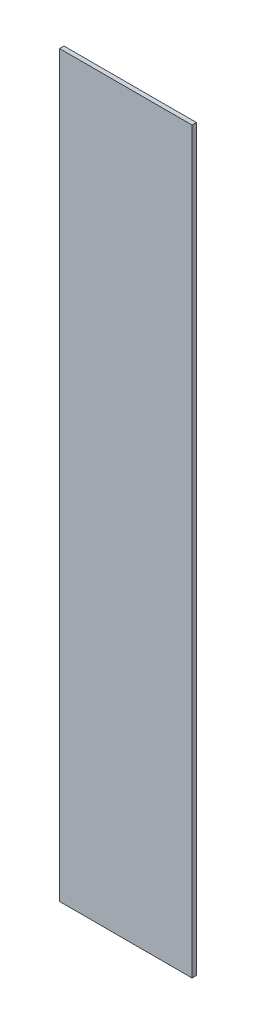
SolidWorks part; units mm, degrees
material "PMMA(有机玻璃)"
ref_plane "前视" through (0, 0, 0) normal (0, 0, 1) x (1, 0, 0)
ref_plane "上视" through (0, 0, 0) normal (0, 1, 0) x (1, 0, 0)
ref_plane "右视" through (0, 0, 0) normal (1, 0, 0) x (0, 0, -1)
sketch "草图1" plane through (0, 0, 0) normal (0, 0, 1) x (1, 0, 0)
  line L1 (-75.5, 421) -> (75.5, 421)
  line L2 (-75.5, 421) -> (-75.5, -421)
  line L3 (-75.5, -421) -> (75.5, -421)
  line L4 (75.5, 421) -> (75.5, -421)
  line L5 (-75.5, 421) -> (75.5, -421) construction
  line L6 (-75.5, -421) -> (75.5, 421) construction
  point P0 (0, 0)
  dimension "D1" = 842
  dimension "D2" = 151
extrude "凸台-拉伸1" add sketch "草图1" along normal blind 5
hole_wizard "M5 间隙孔1" positions "草图3" profile "草图2" hole size "M5" standard "GB"
sketch "草图3" plane through (0, 0, 5) normal (0, 0, 1) x (1, 0, 0)
  line L0 (-427.5, 273) -> (-427.5, -273) construction
  line L1 (-427.5, -273) -> (427.5, -273) construction
  line L2 (0, 273) -> (0, -273) construction
  line L3 (427.5, 273) -> (-427.5, 273) construction
  line L5 (-427.5, 0) -> (427.5, 0) construction
  line L6 (427.5, -273) -> (427.5, 273) construction
  point P0 (-375, -261)
  point P46 (415.5, 250)
  point P48 (-415.5, 250)
  point P58 (-125, -261)
  point P59 (125, -261)
  point P61 (-125, 261)
  point P62 (125, 261)
  point P64 (-375, 261)
  point P88 (375, -261)
  point P89 (375, 261)
  point P108 (415.5, 0)
  point P109 (-415.5, 0)
  point P110 (415.5, -250)
  point P111 (-415.5, -250)
  dimension "D1" = 12
  dimension "D2" = 12
  dimension "D5" = 3
  dimension "D3" = 12
  dimension "D6" = 4
  dimension "D4" = 2
sketch "草图2" plane through (-375, -261, 5) normal (1, 0, 0) x (0, -1, 0)
  line L0 (0, 0) -> (0, 5)
  line L1 (0, 5) -> (2.75, 5)
  line L2 (2.75, 5) -> (2.75, 0)
  line L5 (2.75, 0) -> (0, 0)
  line L11 (0, -6.35) -> (0, 107.95) construction
  dimension "通孔孔直径" = 5.5
  dimension "通孔孔深度" = 5
